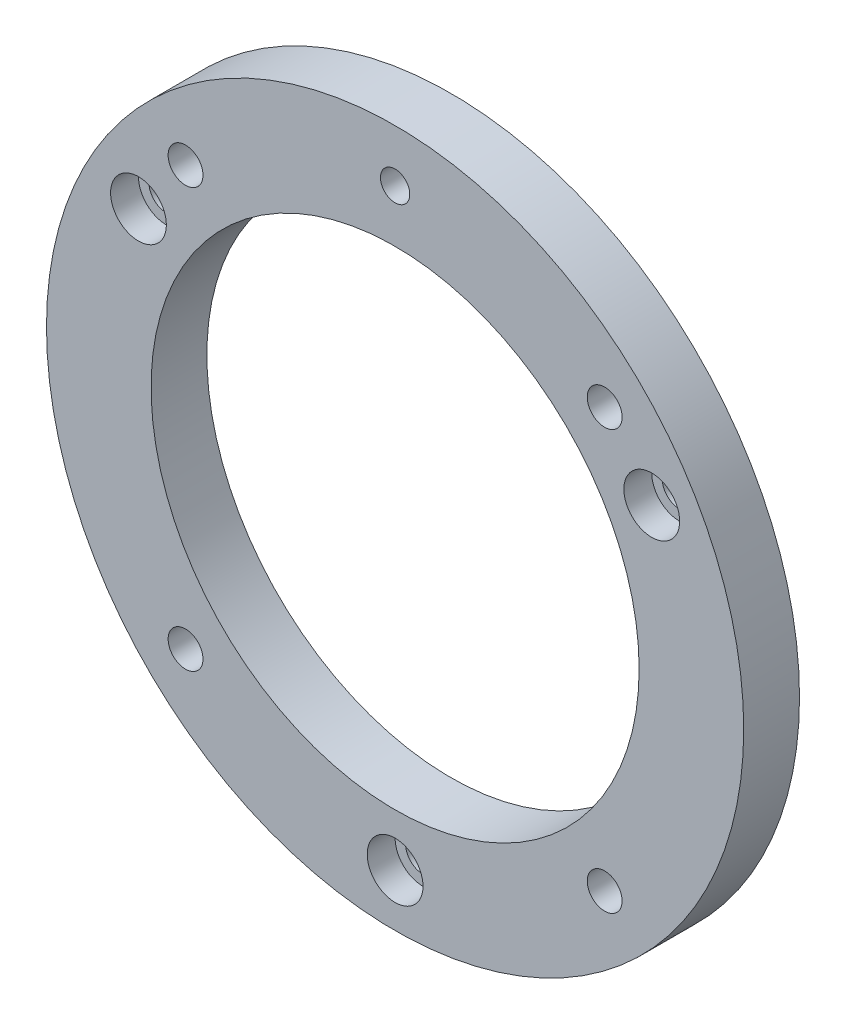
from build123d import *

# Parameters (mm, degrees)
SKETCH1_R           = 50
BOSS_EXTRUDE1_DEPTH = 8
SKETCH2_R           = 2.5
CUT_EXTRUDE1_DEPTH  = 8
SKETCH3_R           = 2.1
CUT_EXTRUDE2_DEPTH  = 8
SKETCH4_R           = 4
CUT_EXTRUDE3_DEPTH  = 4
SKETCH5_R           = 2.5
CUT_EXTRUDE4_DEPTH  = 4
SKETCH6_R           = 35
CUT_EXTRUDE5_DEPTH  = 10


with BuildPart() as part:
    # Sketch1 → Boss-Extrude1 (new body)
    with BuildSketch(Plane.XY):
        Circle(SKETCH1_R)
    extrude(amount=BOSS_EXTRUDE1_DEPTH)

    # Sketch2 → Cut-Extrude1 (cut)
    with BuildSketch(Plane.XY.offset(8)):
        with Locations((-30.054076263, 30.05)):
            Circle(SKETCH2_R)
        with Locations((30.054076263, 30.05)):
            Circle(SKETCH2_R)
        with Locations((-30.054076263, -30.05)):
            Circle(SKETCH2_R)
        with Locations((30.054076263, -30.05)):
            Circle(SKETCH2_R)
    extrude(amount=-CUT_EXTRUDE1_DEPTH, mode=Mode.SUBTRACT)

    # Sketch3 → Cut-Extrude2 (cut)
    with BuildSketch(Plane.XY.offset(8)):
        with Locations((0, 42.5)):
            Circle(SKETCH3_R)
    extrude(amount=-CUT_EXTRUDE2_DEPTH, mode=Mode.SUBTRACT)

    # Sketch4 → Cut-Extrude3 (cut)
    with BuildSketch(Plane.XY.offset(8)):
        with Locations((0, -42.5)):
            Circle(SKETCH4_R)
        with Locations((-36.806079661, 21.25)):
            Circle(SKETCH4_R)
        with Locations((36.806079661, 21.25)):
            Circle(SKETCH4_R)
    extrude(amount=-CUT_EXTRUDE3_DEPTH, mode=Mode.SUBTRACT)

    # Sketch5 → Cut-Extrude4 (cut)
    with BuildSketch(Plane.XY.offset(4)):
        with Locations((-36.806079661, 21.25)):
            Circle(SKETCH5_R)
        with Locations((0, -42.5)):
            Circle(SKETCH5_R)
        with Locations((36.806079661, 21.25)):
            Circle(SKETCH5_R)
    extrude(amount=-CUT_EXTRUDE4_DEPTH, mode=Mode.SUBTRACT)

    # Sketch6 → Cut-Extrude5 (cut)
    with BuildSketch(Plane.XY.offset(8)):
        Circle(SKETCH6_R)
    extrude(amount=-CUT_EXTRUDE5_DEPTH, mode=Mode.SUBTRACT)


solid = part.part
